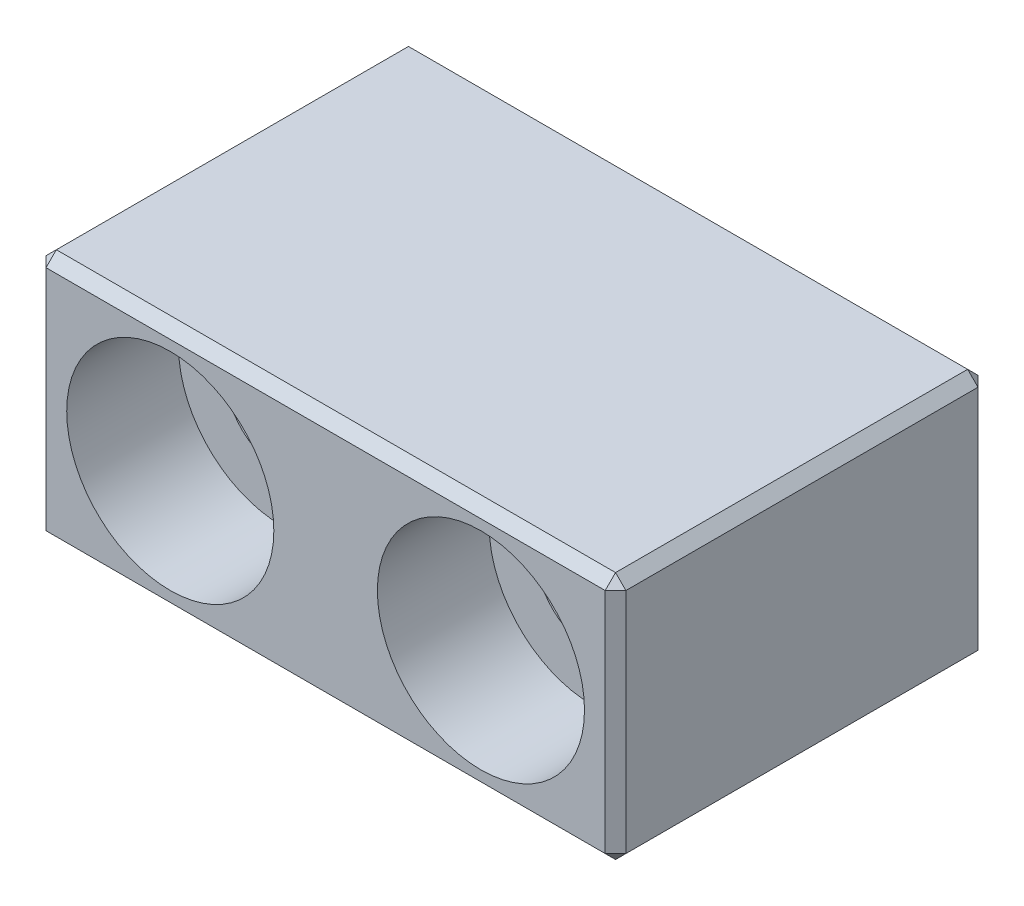
from build123d import *

# Parameters (mm, degrees)
SKETCH_1_W                   = 28
SKETCH_1_H                   = 18
EXTRUDE_1_DEPTH              = 12
HOLE_WIZARD_M5_1_D           = 5.5
HOLE_WIZARD_M5_1_CBORE_D     = 10
HOLE_WIZARD_M5_1_CBORE_DEPTH = 5.4
CHAMFER_1_SIZE               = 0.5


with BuildPart() as part:
    # 草图1 → 凸台-拉伸1 (new body)
    with BuildSketch(Plane(origin=(0, 0, 0), x_dir=(1, 0, 0), z_dir=(0, 1, 0))):
        Rectangle(SKETCH_1_W, SKETCH_1_H)
    extrude(amount=EXTRUDE_1_DEPTH)

    # M5 六角凹头螺钉的柱形沉头孔1 (through all)
    with Locations(Plane.XY.offset(9)):
        with Locations((-7.5, 6), (7.5, 6)):
            CounterBoreHole(HOLE_WIZARD_M5_1_D / 2, HOLE_WIZARD_M5_1_CBORE_D / 2, HOLE_WIZARD_M5_1_CBORE_DEPTH)

    # 倒角1
    chamfer_1_edges = [part.edges().sort_by_distance(p)[0] for p in [
        (-14, 12, 0),
        (0, 12, 9),
        (14, 12, 0),
        (0, 0, 9),
        (-14, 0, 0),
        (0, 0, -9),
        (14, 0, 0),
        (0, 12, -9),
        (14, 6, 9),
        (-14, 6, 9),
        (-14, 6, -9),
        (14, 6, -9),
    ]]
    chamfer(chamfer_1_edges, length=CHAMFER_1_SIZE)


solid = part.part
